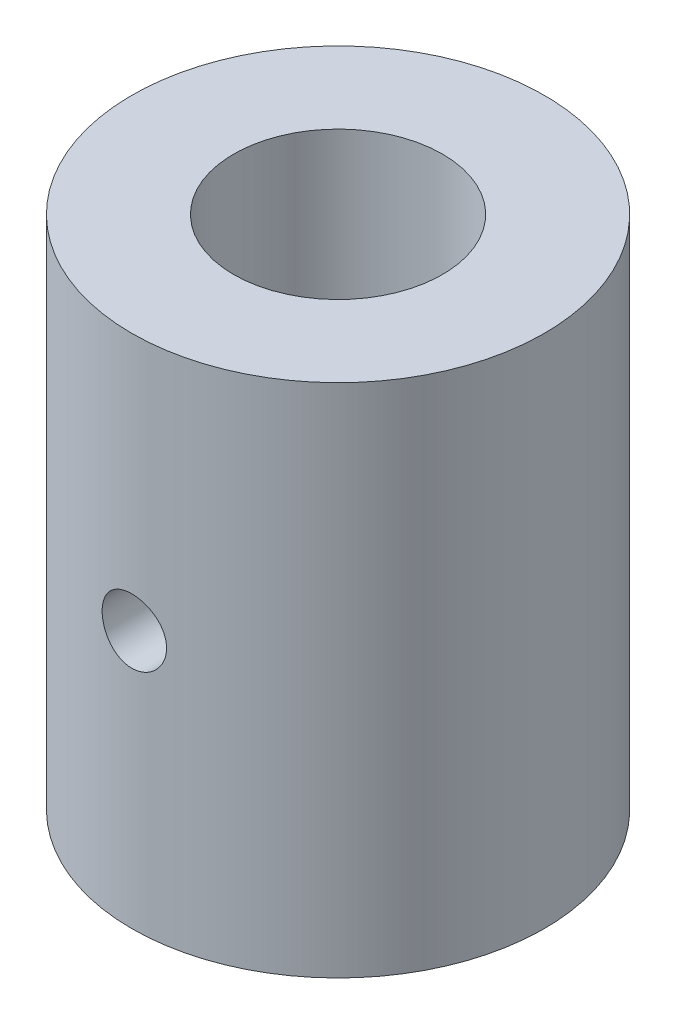
from build123d import *

# Parameters (mm, degrees)
SKETCH1_W              = 3.95
SKETCH1_H              = 20
M3_TAPPED_HOLE1_REACH  = 22.494
M3_TAPPED_HOLE1_BORE_R = 1.25


with BuildPart() as part:
    # Sketch1 → Revolve1 (revolve)
    with BuildSketch(Plane.XY, mode=Mode.PRIVATE) as revolve1_sk:
        with Locations((6.025, 20.516129032)):
            Rectangle(SKETCH1_W, SKETCH1_H)
    revolve(revolve1_sk.sketch.rotate(Axis((0, 29.612903226, 0), (0, -1, 0)), 90), axis=Axis((0, 29.612903226, 0), (0, -1, 0)))

    # M3 Tapped Hole1 bore (on position points) → M3 Tapped Hole1 (cut, up to next)
    with BuildSketch(Plane(origin=(0, 20.516129032, 8), x_dir=(1, 0, 0), z_dir=(0, 0, 1)), mode=Mode.PRIVATE) as m3_tapped_hole1_sk1:
        Circle(M3_TAPPED_HOLE1_BORE_R)
    m3_tapped_hole1_tool1 = extrude(m3_tapped_hole1_sk1.sketch, amount=-M3_TAPPED_HOLE1_REACH, mode=Mode.PRIVATE) & part.part
    add(m3_tapped_hole1_tool1.solids().sort_by_distance((0, 20.516129, 8))[0], mode=Mode.SUBTRACT)


solid = part.part
